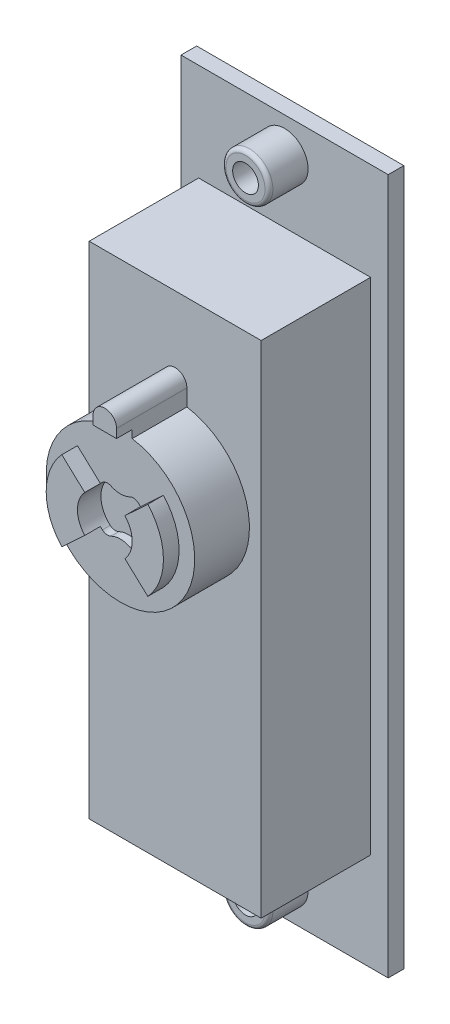
SolidWorks part; units mm, degrees
ref_plane "Front Plane" through (0, 0, 0) normal (0, 0, 1) x (1, 0, 0)
ref_plane "Top Plane" through (0, 0, 0) normal (0, 1, 0) x (1, 0, 0)
ref_plane "Right Plane" through (0, 0, 0) normal (1, 0, 0) x (0, 0, -1)
sketch "Sketch1" plane through (0, 0, 0) normal (0, 0, 1) x (1, 0, 0)
  line L1 (-13.25, -44.5) -> (13.25, -44.5)
  line L2 (-13.25, -44.5) -> (-13.25, 44.5)
  line L3 (-13.25, 44.5) -> (13.25, 44.5)
  line L4 (13.25, -44.5) -> (13.25, 44.5)
  line L5 (-13.25, -44.5) -> (13.25, 44.5) construction
  line L6 (-13.25, 44.5) -> (13.25, -44.5) construction
  point P0 (0, 0)
  dimension "D1" = 89
  dimension "D2" = 26.5
extrude "Boss-Extrude1" add sketch "Sketch1" along normal blind 3
sketch "Sketch2" plane through (0, 0, 3) normal (0, 0, 1) x (1, 0, 0)
  line L1 (-11, -32) -> (11, -32)
  line L2 (-11, -32) -> (-11, 32)
  line L3 (-11, 32) -> (11, 32)
  line L4 (11, -32) -> (11, 32)
  line L5 (-11, -32) -> (11, 32) construction
  line L6 (-11, 32) -> (11, -32) construction
  point P0 (0, 0)
  dimension "D1" = 22
  dimension "D2" = 64
extrude "Boss-Extrude2" add sketch "Sketch2" along normal blind 14
sketch "Sketch3" plane through (0, 0, 3) normal (0, 0, 1) x (1, 0, 0)
  line L0 (0, 0) -> (38.1559, 0) construction
  circle A0 centre (0, 40) radius 3
  circle A1 centre (0, -40) radius 3
  dimension "D1" = 6
  dimension "D2" = 80
extrude "Boss-Extrude3" add sketch "Sketch3" along normal blind 5
hole_wizard "M4 Tapped Hole1" positions "Sketch5" profile "Sketch4" tap size "M4" standard "GB"
sketch "Sketch5" plane through (0, 0, 8) normal (0, 0, 1) x (1, 0, 0)
  point P0 (0, 40)
  point P3 (0, -40)
sketch "Sketch4" plane through (0, 40, 8) normal (1, 0, 0) x (0, -1, 0)
  line L0 (0, 0) -> (0, 5.9914)
  line L1 (0, 5.9914) -> (1.65, 5)
  line L2 (1.65, 5) -> (1.65, 0)
  line L5 (1.65, 0) -> (0, 0)
  line L10 (0, 5.9914) -> (-1.65, 5) construction
  line L11 (0, -6.35) -> (0, 107.95) construction
  dimension "螺纹孔钻头直径" = 3.3
  dimension "螺纹孔钻头深度" = 5
  dimension "导头角度" = 118
cosmetic thread "Cosmetic thread 1" parameters "D1"=5, "D2"=4
cosmetic thread "Cosmetic thread 2" parameters "D1"=5, "D2"=4
chamfer "Chamfer1" distance 3 distance2 1 4 edges at (0, 44.5, 0) (-13.25, 0, 0) (0, -44.5, 0) (13.25, 0, 0)
sketch "Sketch6" plane through (0, 0, 17) normal (0, 0, 1) x (1, 0, 0)
  line L0 (13.25, 44.5) -> (-13.25, 44.5) construction
  circle A0 centre (0, 10.5) radius 9.5
  dimension "D1" = 19
  dimension "D2" = 34
extrude "Boss-Extrude4" add sketch "Sketch6" along normal blind 7
sketch "Sketch7" plane through (0, 0, 17) normal (0, 0, 1) x (1, 0, 0)
  line L0 (0, 21.2176) -> (0, 22) construction
  line L1 (-1.5, 19.8808) -> (-1.5, 22)
  line L2 (1.5, 19.8808) -> (1.5, 22)
  line L3 (-1.5, 19.8808) -> (1.5, 19.8808) construction
  line L4 (-4.3854, 23.5) -> (26.5714, 23.5) construction
  circle A0 centre (0, 10.5) radius 9.5 construction
  arc A1 (1.5, 22) -> (-1.5, 22) centre (0, 22) ccw
  circle A2 centre (0, 10.5) radius 9.5 construction
  arc A3 (-1.5, 19.8808) -> (1.5, 19.8808) centre (0, 10.5) cw
  point P3 (0, 23.1329)
  dimension "D1" = 1.5
  dimension "D3" = 13
extrude "Boss-Extrude5" add sketch "Sketch7" along normal blind 9
sketch "Sketch8" plane through (0, 0, 26) normal (0, 0, 1) x (1, 0, 0)
  line L0 (1.5, 20.8808) -> (-1.5, 20.8808)
  line L1 (1.5, 19.8808) -> (1.5, 22) construction
  line L2 (-1.5, 22) -> (-1.5, 19.8808) construction
  line L3 (-1.5, 20.8808) -> (-1.5, 19.8808)
  line L4 (1.5, 20.8808) -> (1.5, 19.8808)
  arc A1 (1.5, 19.8808) -> (-1.5, 19.8808) centre (0, 10.5) ccw
  arc A2 (-1.5, 19.8808) -> (1.5, 19.8808) centre (0, 10.5) ccw construction
  dimension "D1" = 1
extrude "Cut-Extrude1" cut sketch "Sketch8" against normal up to surface (2 mm away) up to face at (0, 10.5, 24)
sketch "Sketch9" plane through (0, 0, 24) normal (0, 0, 1) x (1, 0, 0)
  circle A0 centre (0, 10.5) radius 7.5
  dimension "D1" = 15
extrude "Boss-Extrude6" add sketch "Sketch9" along normal blind 2
sketch "Sketch12" plane through (0, 0, 26) normal (0, 0, 1) x (1, 0, 0)
  line L0 (0, 10.5) -> (-21.936, 10.5) construction
  line L1 (-3.6308, 13) -> (5.1364, 13) construction
  arc A0 (-2.3055, 13.1333) -> (-2.3055, 7.8667) centre (0, 10.5) ccw
  arc A1 (-1.2077, 13.2794) -> (1.2077, 13.2794) centre (0, 15.75) ccw
  arc A2 (-1.2077, 7.7206) -> (1.2077, 7.7206) centre (0, 5.25) cw
  arc A3 (2.3055, 7.8667) -> (2.3055, 13.1333) centre (0, 10.5) ccw
  arc A4 (-1.2077, 7.7206) -> (-2.3055, 7.8667) centre (-1.6468, 8.619) cw
  arc A5 (1.2077, 7.7206) -> (2.3055, 7.8667) centre (1.6468, 8.619) ccw
  arc A6 (1.2077, 13.2794) -> (2.3055, 13.1333) centre (1.6468, 12.381) cw
  arc A7 (-1.2077, 13.2794) -> (-2.3055, 13.1333) centre (-1.6468, 12.381) ccw
  point P15 (1.6782, 7.4286)
  dimension "D1" = 7
  dimension "D2" = 10.5
  dimension "D3" = 2.5
  dimension "D4" = 1
extrude "Cut-Extrude5" cut sketch "Sketch12" against normal blind 3
sketch "Sketch13" plane through (0, 0, 26) normal (0, 0, 1) x (1, 0, 0)
  line L0 (0, -9.7005) -> (0, 30.7005) construction
  line L1 (2.5667, 12.8795) -> (5.5, 15.599)
  line L2 (-2.5667, 12.8795) -> (-5.5, 15.599)
  line L3 (0, 10.5) -> (16.2159, 10.5) construction
  line L4 (-2.5667, 8.1205) -> (-5.5, 5.401)
  line L5 (2.5667, 8.1205) -> (5.5, 5.401)
  circle A0 centre (0, 10.5) radius 7.5 construction
  arc A1 (-1.2077, 13.2794) -> (-2.3055, 13.1333) centre (-1.6468, 12.381) ccw construction
  arc A2 (-2.3055, 13.1333) -> (-2.3055, 7.8667) centre (0, 10.5) ccw construction
  arc A3 (-1.2077, 13.2794) -> (1.2077, 13.2794) centre (0, 15.75) ccw construction
  arc A4 (2.3055, 13.1333) -> (1.2077, 13.2794) centre (1.6468, 12.381) ccw construction
  arc A5 (2.3055, 7.8667) -> (2.3055, 13.1333) centre (0, 10.5) ccw construction
  arc A6 (-1.2077, 13.2794) -> (-2.3055, 13.1333) centre (-1.6468, 12.381) ccw
  arc A7 (-2.3055, 13.1333) -> (-2.5667, 12.8795) centre (0, 10.5) ccw
  arc A8 (-1.2077, 13.2794) -> (1.2077, 13.2794) centre (0, 15.75) ccw
  arc A9 (2.3055, 13.1333) -> (1.2077, 13.2794) centre (1.6468, 12.381) ccw
  arc A10 (2.5667, 12.8795) -> (2.3055, 13.1333) centre (0, 10.5) ccw
  arc A11 (-5.5, 15.599) -> (5.5, 15.599) centre (0, 10.5) cw
  circle A12 centre (0, 10.5) radius 7.5 construction
  arc A13 (-5.5, 5.401) -> (5.5, 5.401) centre (0, 10.5) ccw
  arc A14 (2.5667, 8.1205) -> (2.3055, 7.8667) centre (0, 10.5) cw
  arc A15 (2.3055, 7.8667) -> (1.2077, 7.7206) centre (1.6468, 8.619) cw
  arc A16 (-1.2077, 7.7206) -> (1.2077, 7.7206) centre (0, 5.25) cw
  arc A17 (-2.3055, 7.8667) -> (-2.5667, 8.1205) centre (0, 10.5) cw
  arc A18 (-1.2077, 7.7206) -> (-2.3055, 7.8667) centre (-1.6468, 8.619) cw
  dimension "D2" = 47.167
  dimension "D1" = 11
extrude "Cut-Extrude6" cut sketch "Sketch13" against normal blind 2
sketch "Sketch14" plane through (0, 0, 0) normal (0, 0, -1) x (-1, 0, 0)
  line L0 (13.25, -44.5) -> (-13.25, -44.5) construction
  circle A0 centre (0, -15.5) radius 6.5
  dimension "D1" = 13
  dimension "D2" = 29
extrude "Boss-Extrude7" add sketch "Sketch14" along normal blind 3
sketch "Sketch15" plane through (0, 0, -3) normal (0, 0, -1) x (-1, 0, 0)
  line L0 (0, -9) -> (0, -22) construction
  line L1 (13.25, -44.5) -> (-13.25, -44.5) construction
  line L2 (1.5, -17) -> (6.3246, -17)
  line L3 (1.5, -17) -> (1.5, -14)
  line L4 (1.5, -14) -> (6.3246, -14)
  line L5 (6.3246, -17) -> (6.3246, -14) construction
  line L6 (1.5, -17) -> (6.3246, -14) construction
  line L7 (1.5, -14) -> (6.3246, -17) construction
  line L8 (-1.5, -14) -> (-6.3246, -17) construction
  line L9 (-1.5, -17) -> (-6.3246, -14) construction
  line L10 (-6.3246, -17) -> (-6.3246, -14) construction
  line L11 (-1.5, -14) -> (-6.3246, -14)
  line L12 (-1.5, -17) -> (-1.5, -14)
  line L13 (-1.5, -17) -> (-6.3246, -17)
  circle A0 centre (0, -15.5) radius 6.5 construction
  circle A1 centre (0, -15.5) radius 6.5 construction
  arc A2 (6.3246, -17) -> (6.3246, -14) centre (0, -15.5) ccw
  arc A3 (-6.3246, -17) -> (-6.3246, -14) centre (0, -15.5) cw
  point P5 (3.9123, -15.5)
  point P16 (-3.9123, -15.5)
  dimension "D1" = 29
  dimension "D2" = 3
  dimension "D3" = 4.8246
extrude "Cut-Extrude7" cut sketch "Sketch15" against normal blind 2.5
fillet "Fillet1" radius 1 8 edges at (1.5, -15.5, -3) (3.9123, -14, -3) (0, -9, -3) (-3.9123, -14, -3) (-1.5, -15.5, -3) (-3.9123, -17, -3) (0, -22, -3) (3.9123, -17, -3)
sketch "Sketch16" plane through (0, 0, 0) normal (0, 0, -1) x (-1, 0, 0)
  line L0 (0, 0) -> (0, 54.5365) construction
  line L1 (-2.8227, 32.6593) -> (-8.6342, 16.5162)
  line L2 (-8.6342, 14.4838) -> (-2.8227, -1.6593)
  line L3 (8.6342, 14.4838) -> (2.8227, -1.6593)
  line L4 (2.8227, 32.6593) -> (8.6342, 16.5162)
  line L5 (13.25, -44.5) -> (-13.25, -44.5) construction
  arc A0 (-2.8227, -1.6593) -> (2.8227, -1.6593) centre (0, -0.6431) ccw
  arc A1 (8.6342, 14.4838) -> (8.6342, 16.5162) centre (5.8115, 15.5) ccw
  arc A2 (-8.6342, 16.5162) -> (-8.6342, 14.4838) centre (-5.8115, 15.5) ccw
  arc A3 (-2.8227, 32.6593) -> (2.8227, 32.6593) centre (0, 31.6431) cw
  point P9 (0, -9.5)
  point P12 (9, 15.5)
  point P15 (-9, 15.5)
  point P18 (0, 40.5)
  dimension "D3" = 3
  dimension "D1" = 50
  dimension "D2" = 18
  dimension "D4" = 60
extrude "Boss-Extrude8" add sketch "Sketch16" along normal blind 3
fillet "Fillet2" radius 1 8 edges at (5.7284, 6.4123, -3) (8.8115, 15.5, -3) (5.7284, 24.5877, -3) (0, 34.6431, -3) (-5.7284, 24.5877, -3) (-8.8115, 15.5, -3) (-5.7284, 6.4123, -3) (0, -3.6431, -3)
fillet "Fillet3" radius 0.5 2 edges at (-3, -40, 8) (3, 40, 8)
